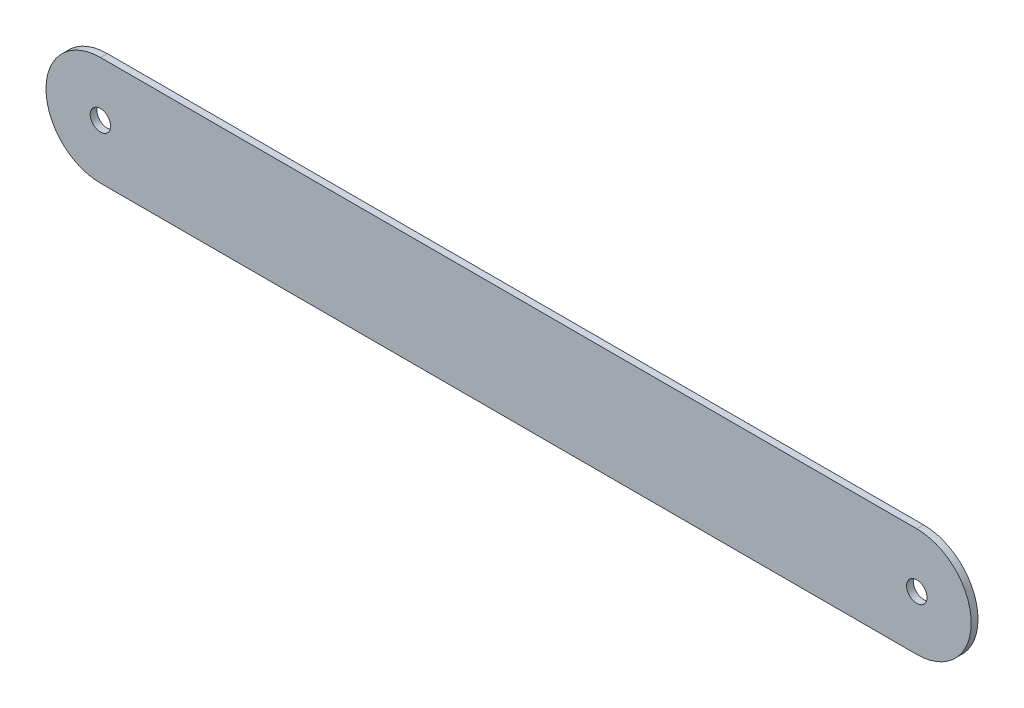
from build123d import *

# Parameters (mm, degrees)
EXTRUDE_1_DEPTH     = 5
SKETCH_2_R          = 7.5
CUT_EXTRUDE_1_DEPTH = 642.268274593


with BuildPart() as part:
    # 草图1 → 凸台-拉伸1 (new body)
    with BuildSketch(Plane.XY):
        with BuildLine():
            Line((0, 40), (600, 40))
            ThreePointArc((600, 40), (640, 0), (600, -40))
            Line((600, -40), (0, -40))
            ThreePointArc((0, -40), (-40, 0), (0, 40))
        make_face()
    extrude(amount=EXTRUDE_1_DEPTH)

    # 草图2 → 切除-拉伸1 (cut, through all)
    with BuildSketch(Plane.XY.offset(5)):
        Circle(SKETCH_2_R)
        with Locations((600, 0)):
            Circle(SKETCH_2_R)
    extrude(amount=-CUT_EXTRUDE_1_DEPTH, mode=Mode.SUBTRACT)


solid = part.part
